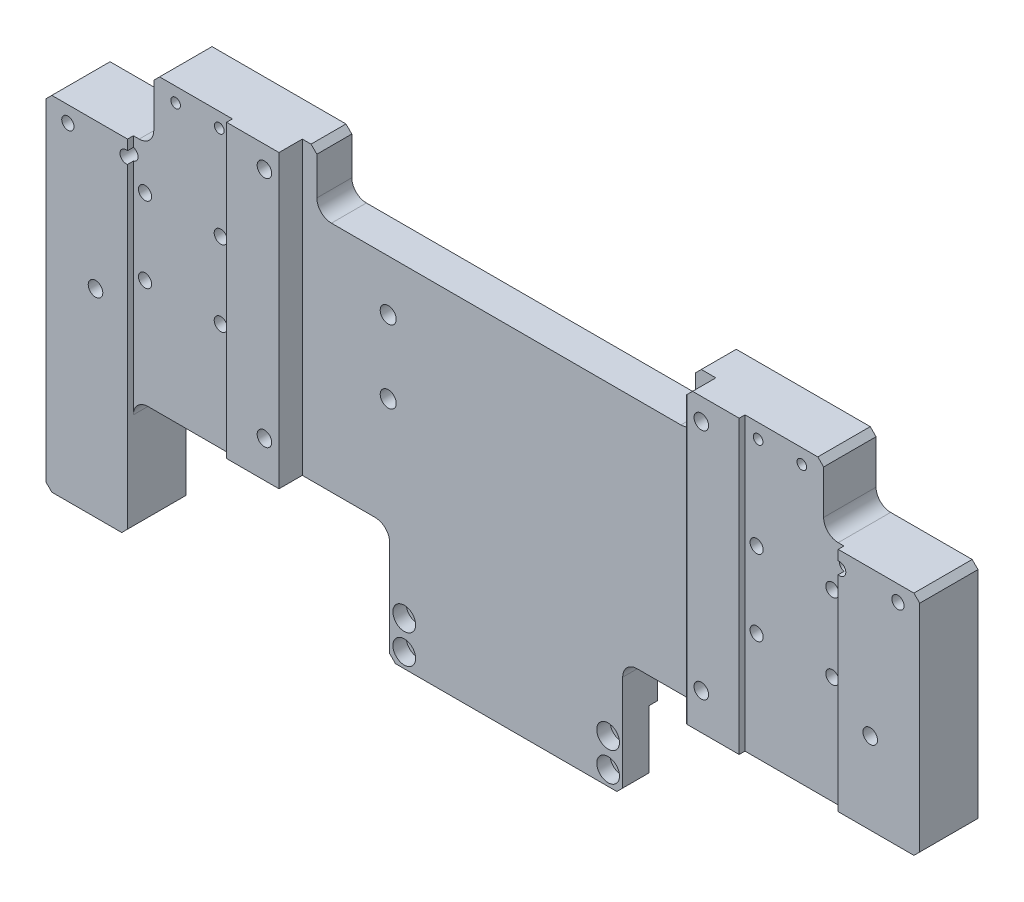
from build123d import *

# Parameters (mm, degrees)
SKETCH_1_W                   = 300
SKETCH_1_H                   = 100
EXTRUDE_1_DEPTH              = 20
CHAMFER_1_SIZE               = 2
SKETCH_2_W                   = 34
SKETCH_2_H                   = 2
CUT_EXTRUDE_1_DEPTH          = 182.383571472
SKETCH_3_W                   = 140
SKETCH_3_H                   = 8
CUT_EXTRUDE_2_DEPTH          = 182.383571472
SKETCH_4_W                   = 80
SKETCH_4_H                   = 40
EXTRUDE_2_DEPTH              = 12
FILLET_1_R                   = 5
SKETCH_5_W                   = 3
SKETCH_5_H                   = 22
CUT_EXTRUDE_3_DEPTH          = 212.187120819
CHAMFER_2_SIZE               = 2
SKETCH_6_W                   = 130
SKETCH_6_H                   = 20
CUT_EXTRUDE_4_DEPTH          = 177.068168617
FILLET_2_R                   = 5
HOLE_WIZARD_M6_1_D           = 5
SKETCH_10_W                  = 35
SKETCH_10_H                  = 22
CUT_EXTRUDE_5_DEPTH          = 177.068168617
CHAMFER_3_SIZE               = 2
FILLET_3_R                   = 5
HOLE_WIZARD_M5_1_D           = 5.5
HOLE_WIZARD_M5_1_CBORE_D     = 10
HOLE_WIZARD_M5_1_CBORE_DEPTH = 5.7
HOLE_WIZARD_M4_1_D           = 4.5
HOLE_WIZARD_M4_1_CBORE_D     = 8
HOLE_WIZARD_M4_1_CBORE_DEPTH = 4.6
HOLE_WIZARD_M6_2_D           = 5
HOLE_WIZARD_M3_1_D           = 2.5
HOLE_WIZARD_M3_1_DEPTH       = 7.5
HOLE_WIZARD_M3_1_TIP         = 0.751075774
HOLE_WIZARD_M5_1_2_D         = 4.2
HOLE_WIZARD_M4_3_D           = 4.5
HOLE_WIZARD_M4_3_CBORE_D     = 7.8
HOLE_WIZARD_M4_3_CBORE_DEPTH = 4.6
CHAMFER_4_SIZE               = 2
SKETCH_31_W                  = 28
SKETCH_31_H                  = 20
EXTRUDE_3_DEPTH              = 40
CHAMFER_5_SIZE               = 2
FILLET_4_R                   = 5
HOLE_WIZARD_M4_1_2_D         = 3.3


with BuildPart() as part:
    # 草图1 → 凸台-拉伸1 (new body)
    with BuildSketch(Plane.XY):
        Rectangle(SKETCH_1_W, SKETCH_1_H)
    extrude(amount=EXTRUDE_1_DEPTH)

    # 倒角1
    chamfer_1_edges = [part.edges().sort_by_distance(p)[0] for p in [
        (150, -50, 10),
        (150, 50, 10),
        (-150, 50, 10),
    ]]
    chamfer(chamfer_1_edges, length=CHAMFER_1_SIZE)

    # 草图2 → 切除-拉伸1 (cut, through all)
    with BuildSketch(Plane.XZ.offset(50)):
        with Locations((-105, 19)):
            Rectangle(SKETCH_2_W, SKETCH_2_H)
        with Locations((105, 19)):
            Rectangle(SKETCH_2_W, SKETCH_2_H)
    extrude(amount=-CUT_EXTRUDE_1_DEPTH, mode=Mode.SUBTRACT)

    # 草图3 → 切除-拉伸2 (cut, through all)
    with BuildSketch(Plane.XZ.offset(50)):
        with Locations((0, 16)):
            Rectangle(SKETCH_3_W, SKETCH_3_H)
    extrude(amount=-CUT_EXTRUDE_2_DEPTH, mode=Mode.SUBTRACT)

    # 草图4 → 凸台-拉伸2 (add)
    with BuildSketch(Plane(origin=(0, 0, 0), x_dir=(-1, 0, 0), z_dir=(0, 0, -1))):
        with Locations((0, -70)):
            Rectangle(SKETCH_4_W, SKETCH_4_H)
    extrude(amount=-EXTRUDE_2_DEPTH)

    # 圆角1
    fillet_1_edges = [part.edges().sort_by_distance(p)[0] for p in [
        (40, -50, 6),
        (-40, -50, 6),
    ]]
    fillet(fillet_1_edges, radius=FILLET_1_R)

    # 草图5 → 切除-拉伸3 (cut, through all)
    with BuildSketch(Plane(origin=(40, 0, 0), x_dir=(0, 0, -1), z_dir=(1, 0, 0))):
        with Locations((-1.5, -79)):
            Rectangle(SKETCH_5_W, SKETCH_5_H)
    extrude(amount=-CUT_EXTRUDE_3_DEPTH, mode=Mode.SUBTRACT)

    # 倒角2
    chamfer_2_edges = [part.edges().sort_by_distance(p)[0] for p in [
        (40, -90, 7.5),
        (-40, -90, 7.5),
    ]]
    chamfer(chamfer_2_edges, length=CHAMFER_2_SIZE)

    # 草图6 → 切除-拉伸4 (cut, through all)
    with BuildSketch(Plane(origin=(0, 0, 0), x_dir=(-1, 0, 0), z_dir=(0, 0, -1))):
        with Locations((0, 40)):
            Rectangle(SKETCH_6_W, SKETCH_6_H)
    extrude(amount=-CUT_EXTRUDE_4_DEPTH, mode=Mode.SUBTRACT)

    # 圆角2
    fillet_2_edges = [part.edges().sort_by_distance(p)[0] for p in [
        (65, 30, 6),
        (-65, 30, 6),
    ]]
    fillet(fillet_2_edges, radius=FILLET_2_R)

    # M6 螺纹孔1 (through all)
    with Locations(Plane(origin=(0, 0, 0), x_dir=(-1, 0, 0), z_dir=(0, 0, -1))):
        with Locations((133, -22), (-133, -22)):
            Hole(HOLE_WIZARD_M6_1_D / 2)

    # 草图10 → 切除-拉伸5 (cut, through all)
    with BuildSketch(Plane(origin=(0, 0, 0), x_dir=(-1, 0, 0), z_dir=(0, 0, -1))):
        with Locations((132.5, 39)):
            Rectangle(SKETCH_10_W, SKETCH_10_H)
        with Locations((-132.5, 39)):
            Rectangle(SKETCH_10_W, SKETCH_10_H)
    extrude(amount=-CUT_EXTRUDE_5_DEPTH, mode=Mode.SUBTRACT)

    # 倒角3
    chamfer_3_edges = [part.edges().sort_by_distance(p)[0] for p in [
        (-150, 28, 10),
        (-115, 50, 9),
        (115, 50, 9),
        (150, 28, 10),
        (70, 50, 16),
    ]]
    chamfer(chamfer_3_edges, length=CHAMFER_3_SIZE)

    # 圆角3
    fillet_3_edges = [part.edges().sort_by_distance(p)[0] for p in [
        (-115, 28, 9),
        (115, 28, 9),
    ]]
    fillet(fillet_3_edges, radius=FILLET_3_R)

    # Hole Wizard M5 _1 (through all)
    with Locations(Plane(origin=(0, 0, 0), x_dir=(-1, 0, 0), z_dir=(0, 0, -1))):
        with Locations((40.5, 12.5), (40.5, -12.5)):
            CounterBoreHole(HOLE_WIZARD_M5_1_D / 2, HOLE_WIZARD_M5_1_CBORE_D / 2, HOLE_WIZARD_M5_1_CBORE_DEPTH)

    # Hole Wizard M4 _1 (through all)
    with Locations(Plane(origin=(0, 0, 0), x_dir=(-1, 0, 0), z_dir=(0, 0, -1))):
        with Locations((92, 13), (118, 13), (118, -13), (92, -13), (-92, -13), (-118, -13), (-118, 13), (-92, 13)):
            CounterBoreHole(HOLE_WIZARD_M4_1_D / 2, HOLE_WIZARD_M4_1_CBORE_D / 2, HOLE_WIZARD_M4_1_CBORE_DEPTH)

    # M6 螺纹孔2 (through all)
    with Locations(Plane(origin=(0, 0, 0), x_dir=(-1, 0, 0), z_dir=(0, 0, -1))):
        with Locations((75, 42.5), (75, -37.5), (-75, -37.5), (-75, 42.5)):
            Hole(HOLE_WIZARD_M6_2_D / 2)

    # M3 螺纹孔1
    with Locations(Plane(origin=(0, 0, 0), x_dir=(-1, 0, 0), z_dir=(0, 0, -1))):
        with Locations((19.5, 20), (19.5, -10), (-19.5, -10), (-19.5, 20)):
            Hole(HOLE_WIZARD_M3_1_D / 2, depth=HOLE_WIZARD_M3_1_DEPTH)
            with Locations((0, 0, -(HOLE_WIZARD_M3_1_DEPTH + HOLE_WIZARD_M3_1_TIP / 2))):  # 118° drill point
                Cone(0, HOLE_WIZARD_M3_1_D / 2, HOLE_WIZARD_M3_1_TIP, mode=Mode.SUBTRACT)

    # Hole Wizard M5 _1 2 (through all)
    with Locations(Plane(origin=(0, 0, 0), x_dir=(-1, 0, 0), z_dir=(0, 0, -1))):
        with Locations((-142.5, 22.5), (-122.5, 22.5), (122.5, 22.5), (142.5, 22.5)):
            Hole(HOLE_WIZARD_M5_1_2_D / 2)

    # M4 六角圆柱头螺钉的柱形沉头孔3 (through all)
    with Locations(Plane.XY.offset(12)):
        with Locations((-35, -75), (-35, -85), (35, -75), (35, -85)):
            CounterBoreHole(HOLE_WIZARD_M4_3_D / 2, HOLE_WIZARD_M4_3_CBORE_D / 2, HOLE_WIZARD_M4_3_CBORE_DEPTH)

    # 倒角4
    chamfer_4_edges = [part.edges().sort_by_distance(p)[0] for p in [
        (65, 50, 6),
        (-65, 50, 6),
    ]]
    chamfer(chamfer_4_edges, length=CHAMFER_4_SIZE)

    # 草图31 → 凸台-拉伸3 (add)
    with BuildSketch(Plane.XZ.offset(50)):
        with Locations((-136, 10)):
            Rectangle(SKETCH_31_W, SKETCH_31_H)
    extrude(amount=EXTRUDE_3_DEPTH)

    # 倒角5
    chamfer_5_edges = [part.edges().sort_by_distance(p)[0] for p in [
        (-150, -90, 10),
        (-122, -90, 10),
    ]]
    chamfer(chamfer_5_edges, length=CHAMFER_5_SIZE)

    # 圆角4
    fillet_4_edges = [part.edges().sort_by_distance(p)[0] for p in [
        (-122, -50, 9),
    ]]
    fillet(fillet_4_edges, radius=FILLET_4_R)

    # Hole Wizard M4 _1 2 (through all)
    with Locations(Plane(origin=(0, 0, 0), x_dir=(-1, 0, 0), z_dir=(0, 0, -1))):
        with Locations((-107.5, 45), (-92.5, 45), (92.5, 45), (107.5, 45)):
            Hole(HOLE_WIZARD_M4_1_2_D / 2)


solid = part.part
